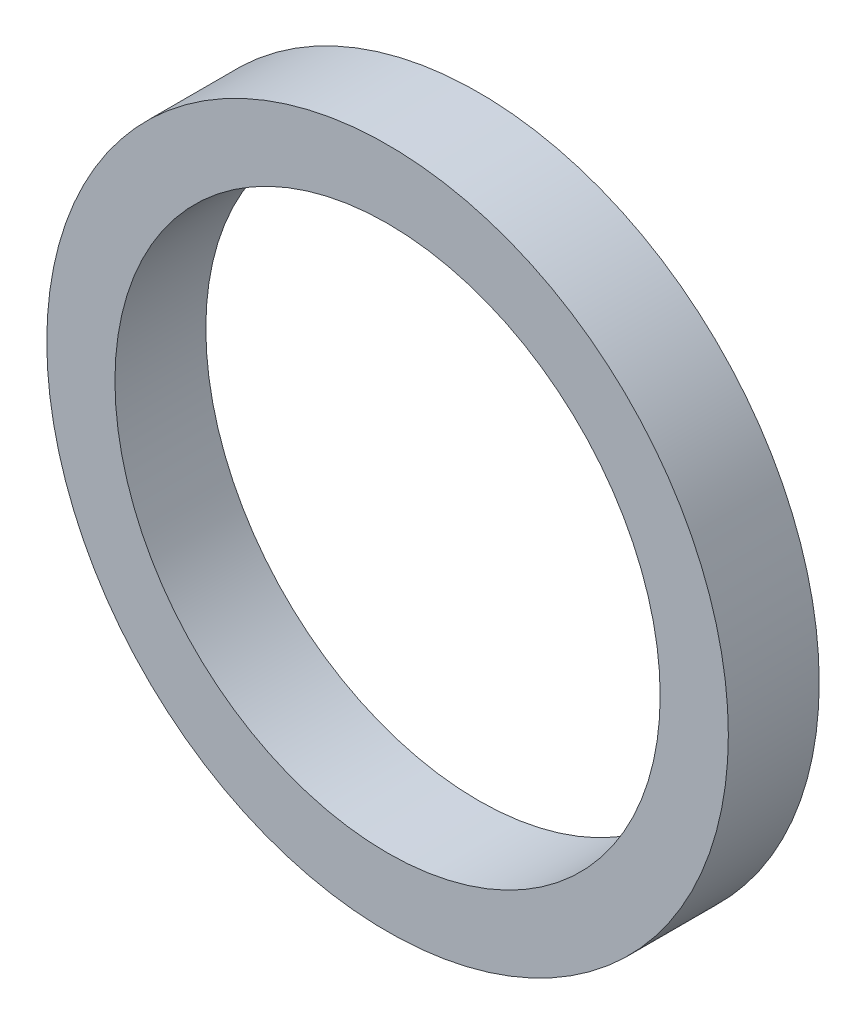
from build123d import *

# Parameters (mm, degrees)
SKETCH2_R           = 7.5
SKETCH2_R_2         = 6
BOSS_EXTRUDE1_DEPTH = 2


with BuildPart() as part:
    # Sketch2 → Boss-Extrude1 (new body)
    with BuildSketch(Plane.XY):
        Circle(SKETCH2_R)
        Circle(SKETCH2_R_2, mode=Mode.SUBTRACT)
    extrude(amount=BOSS_EXTRUDE1_DEPTH)


solid = part.part
